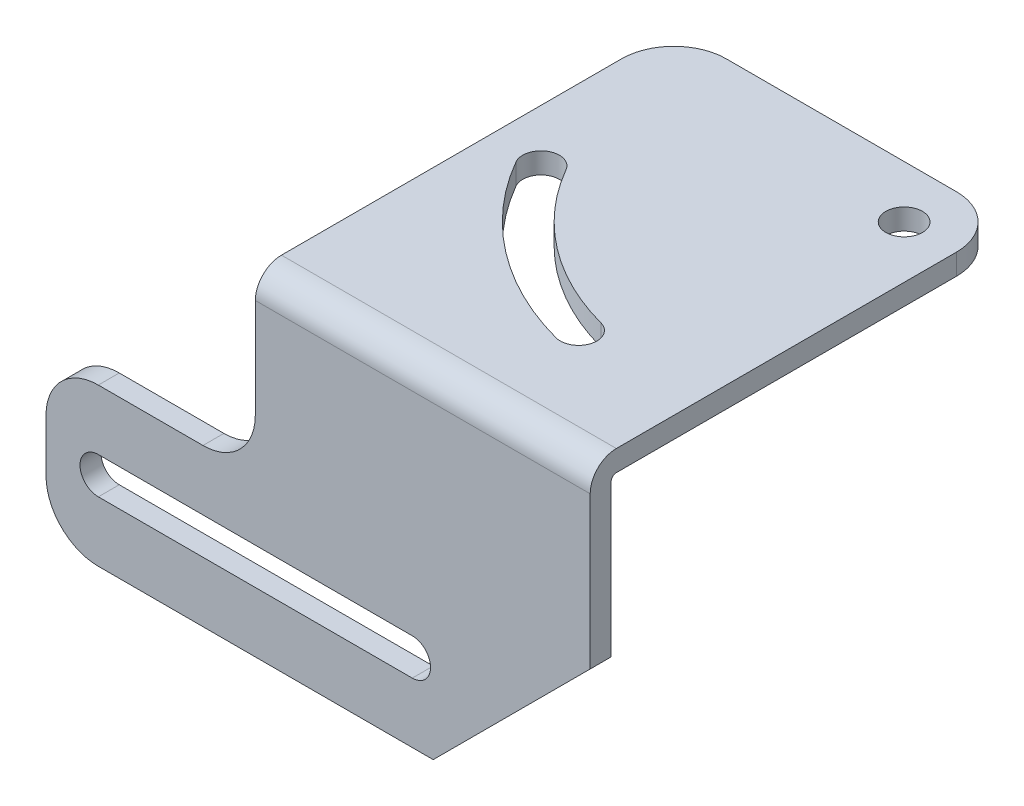
SolidWorks part; units mm, degrees
material "2.0不锈钢"
ref_plane "Front" through (0, 0, 0) normal (0, 0, 1) x (1, 0, 0)
ref_plane "Top" through (0, 0, 0) normal (0, 1, 0) x (1, 0, 0)
ref_plane "Right" through (0, 0, 0) normal (1, 0, 0) x (0, 0, -1)
ref_plane "基准面1" through (0, 0, 0) normal (-1, 0, 0) x (0, -1, 0)
sketch "草图1" plane through (0, 0, 0) normal (-1, 0, 0) x (0, -1, 0)
  line L0 (8, -50) -> (40, -50)
  line L1 (40, -50) -> (40, -10)
  line L2 (40, -10) -> (8, -10)
  line L3 (8, -10) -> (8, -50)
  dimension "D1" = 32
  dimension "D2" = 40
extrude "凸台-拉伸1" add sketch "草图1" against normal blind 32
sketch "草图2" plane through (32, 0, 0) normal (1, 0, 0) x (0, 0, -1)
  line L0 (57.5899, -45.822) -> (57.5899, -10)
  line L1 (57.5899, -10) -> (12, -10)
  line L2 (12, -10) -> (12, -45.822)
  line L3 (12, -45.822) -> (57.5899, -45.822)
  line L4 (10, -8) -> (50, -8) construction
  line L5 (10, -40) -> (10, -8) construction
  dimension "D1" = 2
  dimension "D2" = 2
extrude "切除-拉伸1" cut sketch "草图2" against normal through all
hole_wizard "Ø3.5 (3.5) 直径孔1" positions "草图6" profile "草图5" hole size "Ø3.5" standard "Ansi Metric" end condition through all
sketch "草图6" plane through (0, -10, 0) normal (0, -1, 0) x (-1, 0, 0)
  line L5 (-32, 10) -> (-32, 50) construction
  line L6 (0, 50) -> (-32, 50) construction
  line L7 (-27, 45) -> (-5.003, 32.3) construction
  line L9 (-27, 45) -> (-12.8455, 45) construction
  point P0 (-5.003, 32.3)
  point P1 (-27, 45)
  dimension "D1" = 25.4
  dimension "D2" = 5
  dimension "D3" = 5
  dimension "D4" = 30
sketch "草图5" plane through (5.003, -10, -32.3) normal (1, 0, 0) x (0, 0, -1)
  line L0 (0, 0) -> (0, 2)
  line L1 (0, 2) -> (1.75, 2)
  line L2 (1.75, 2) -> (1.75, 0)
  line L5 (1.75, 0) -> (0, 0)
  line L11 (0, -6.35) -> (0, 107.95) construction
  dimension "通孔孔直径" = 3.5
  dimension "通孔孔深度" = 2
fillet "圆角1" radius 0.5 1 edges at (16, -10, -12)
fillet "圆角3" radius 2.5 1 edges at (16, -8, -10)
sketch "草图8" plane through (0, -8, 0) normal (0, 1, 0) x (1, 0, 0)
  line L0 (27, 45) -> (5.003, 32.3) construction
  line L2 (20.426, 20.4655) -> (27, 45) construction
  circle A0 centre (27, 45) radius 25.4 construction
  arc A1 (5.003, 32.3) -> (20.426, 20.4655) centre (27, 45) ccw construction
  arc A2 (3.4874, 31.425) -> (19.9731, 18.7751) centre (27, 45) ccw
  arc A3 (6.5185, 33.175) -> (20.8789, 22.1559) centre (27, 45) ccw
  arc A4 (6.5185, 33.175) -> (3.4874, 31.425) centre (5.003, 32.3) ccw
  arc A5 (19.9731, 18.7751) -> (20.8789, 22.1559) centre (20.426, 20.4655) ccw
  circle A7 centre (5.003, 32.3) radius 1.75 construction
  point P6 (11.5375, 24.8488)
  dimension "D1" = 45
extrude "切除-拉伸3" cut sketch "草图8" against normal up to next
sketch "草图9" plane through (0, 0, 0) normal (-1, 0, 0) x (0, 0, 1)
  line L0 (-12, -10.5) -> (-12, -40) construction
  line L1 (-10, -40) -> (-12, -40)
  line L2 (-10, -40) -> (-10, -25)
  line L3 (-10, -25) -> (-12, -25)
  line L4 (-12, -40) -> (-12, -25)
  dimension "D1" = 15
extrude "凸台-拉伸2" add sketch "草图9" along normal blind 20
sketch "草图10" plane through (0, 0, -12) normal (0, 0, -1) x (-1, 0, 0)
  line L0 (-15, -32.5) -> (15, -32.5) construction
  line L1 (-15, -30.75) -> (15, -30.75)
  line L2 (-15, -34.25) -> (15, -34.25)
  line L3 (20, -25) -> (0, -25) construction
  line L4 (20, -25) -> (20, -40) construction
  arc A0 (-15, -30.75) -> (-15, -34.25) centre (-15, -32.5) ccw
  arc A1 (15, -34.25) -> (15, -30.75) centre (15, -32.5) ccw
  point P2 (0, -32.5)
  dimension "D2" = 5
  dimension "D3" = 1.75
  dimension "D1" = 7.5
  dimension "D4" = 30
extrude "切除-拉伸4" cut sketch "草图10" against normal through all
chamfer "倒角1" distance 15 angle 45 1 edges at (32, -40, -11)
fillet "圆角4" radius 5 5 edges at (-20, -40, -11) (-20, -25, -11) (0, -9, -50) (32, -9, -50)
